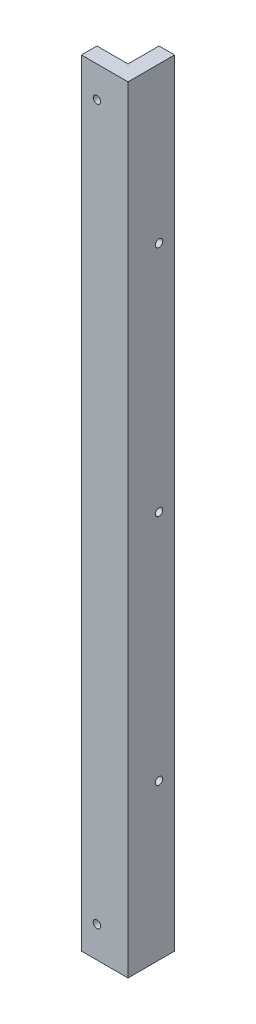
SolidWorks part; units mm, degrees
ref_plane "Front Plane" through (0, 0, 0) normal (0, 0, 1) x (1, 0, 0)
ref_plane "Top Plane" through (0, 0, 0) normal (0, 1, 0) x (1, 0, 0)
ref_plane "Right Plane" through (0, 0, 0) normal (1, 0, 0) x (0, 0, -1)
sketch "Sketch1" plane through (0, 0, 0) normal (0, 1, 0) x (1, 0, 0)
  line L0 (0, 0) -> (15, 0)
  line L1 (15, 0) -> (15, 15)
  line L2 (15, 15) -> (10, 15)
  line L3 (10, 15) -> (10, 5)
  line L4 (10, 5) -> (0, 5)
  line L5 (0, 5) -> (0, 0)
  dimension "D1" = 5
  dimension "D2" = 15
  dimension "D3" = 10
  dimension "D4" = 15
extrude "Boss-Extrude1" add sketch "Sketch1" along normal blind 250
sketch "Sketch2" plane through (15, 0, 0) normal (1, 0, 0) x (0, 0, -1)
  line L0 (10, 10) -> (10, 240) construction
  line L2 (0, 250) -> (0, 0) construction
  line L3 (0, 250) -> (15, 250) construction
  line L4 (0, 0) -> (15, 0) construction
  dimension "D1" = 10
  dimension "D2" = 10
  dimension "D3" = 10
sketch "Sketch3" plane through (10, 0, 0) normal (-1, 0, 0) x (0, 0, 1)
  circle A0 centre (-10, 50) radius 1.2
  circle A1 centre (-10, 125) radius 1.2
  circle A2 centre (-10, 200) radius 1.2
extrude "Cut-Extrude1" cut sketch "Sketch3" against normal blind 10
sketch "Sketch4" plane through (0, 0, 0) normal (0, 0, 1) x (1, 0, 0)
  circle A0 centre (5, 10) radius 1.2
  circle A1 centre (5, 240) radius 1.2
extrude "Cut-Extrude2" cut sketch "Sketch4" against normal blind 5
